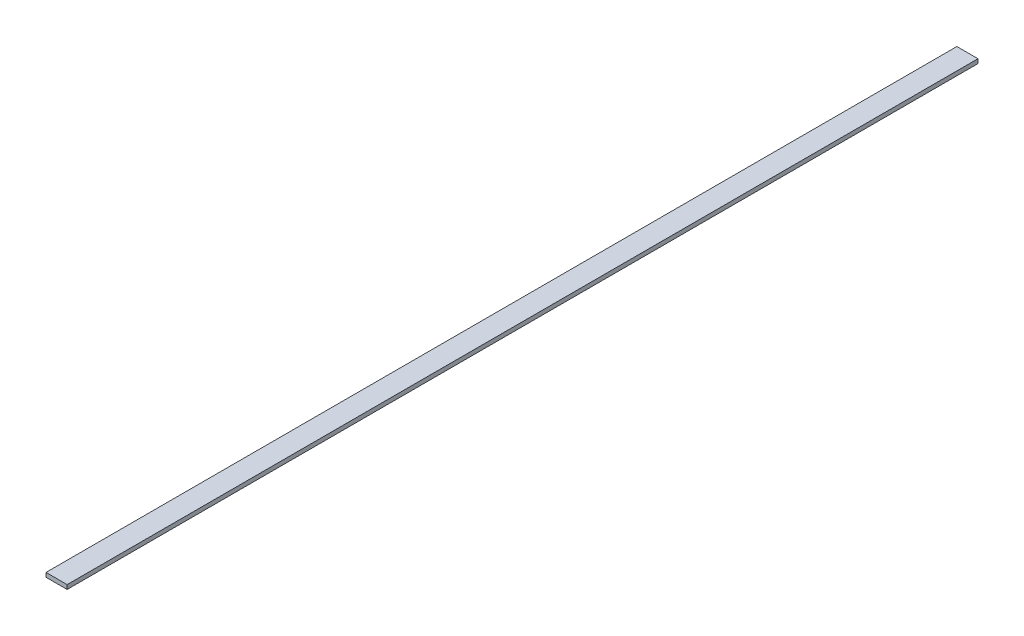
SolidWorks part; units mm, degrees
ref_plane "Front Plane" through (0, 0, 0) normal (0, 0, 1) x (1, 0, 0)
ref_plane "Top Plane" through (0, 0, 0) normal (0, 1, 0) x (1, 0, 0)
ref_plane "Right Plane" through (0, 0, 0) normal (1, 0, 0) x (0, 0, -1)
other "Configuration Table"
sketch "Sketch1" plane through (0, 0, 0) normal (0, 0, 1) x (1, 0, 0)
  line L1 (-35, 7) -> (35, 7)
  line L2 (-35, 7) -> (-35, -7)
  line L3 (-35, -7) -> (35, -7)
  line L4 (35, 7) -> (35, -7)
  line L5 (-35, 7) -> (35, -7) construction
  line L6 (-35, -7) -> (35, 7) construction
  point P0 (0, 0)
  dimension "D1" = 70
  dimension "D2" = 14
extrude "Boss-Extrude1" add sketch "Sketch1" along normal blind 3017.15
